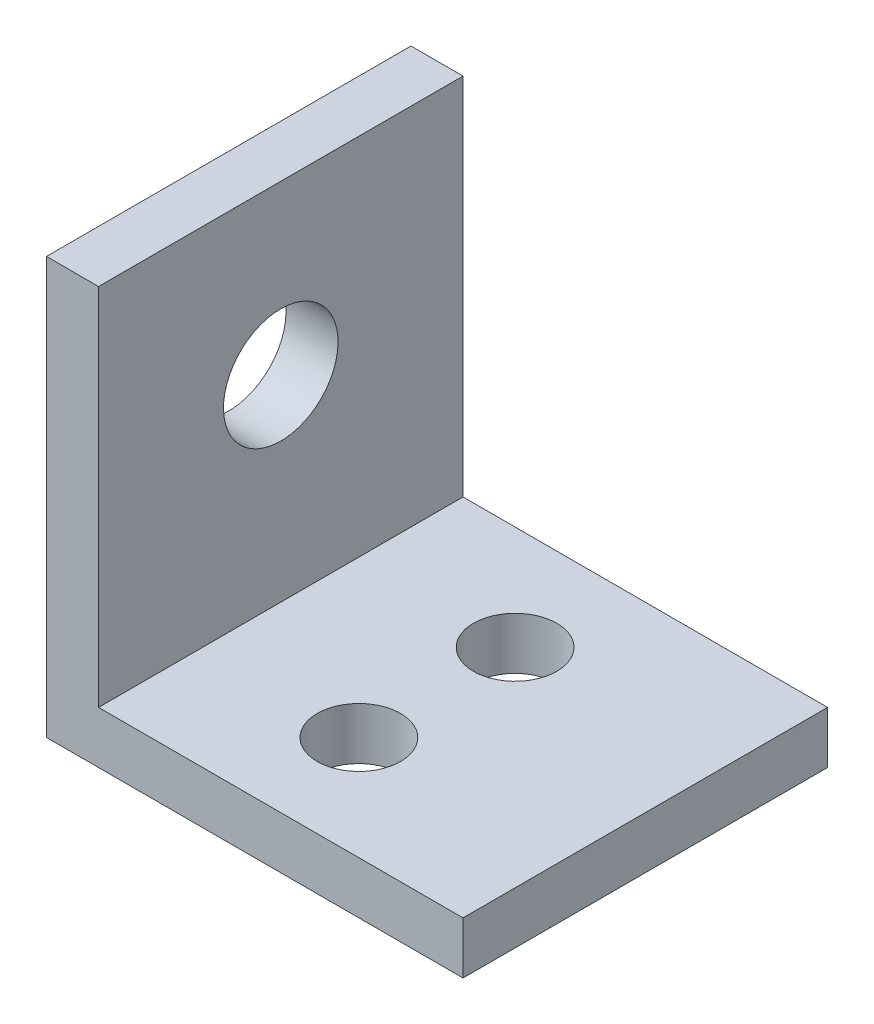
from build123d import *

# Parameters (mm, degrees)
BOSS_EXTRUDE1_DEPTH = 70
SKETCH2_R           = 8
CUT_EXTRUDE1_DEPTH  = 90
SKETCH3_R           = 11
CUT_EXTRUDE2_DEPTH  = 90


with BuildPart() as part:
    # Sketch1 → Boss-Extrude1 (new body)
    with BuildSketch(Plane.XY):
        Polygon((0, 0), (0, 80), (10, 80), (10, 10), (80, 10), (80, 0), align=None)
    extrude(amount=BOSS_EXTRUDE1_DEPTH)

    # Sketch2 → Cut-Extrude1 (cut)
    with BuildSketch(Plane(origin=(0, 10, 0), x_dir=(1, 0, 0), z_dir=(0, 1, 0))):
        with Locations(Location((40, -20, 0), (0, 0, 270))):
            Circle(SKETCH2_R)
        with Locations(Location((40, -50, 0), (0, 0, 270))):
            Circle(SKETCH2_R)
    extrude(amount=-CUT_EXTRUDE1_DEPTH, mode=Mode.SUBTRACT)

    # Sketch3 → Cut-Extrude2 (cut)
    with BuildSketch(Plane(origin=(10, 0, 0), x_dir=(0, 0, -1), z_dir=(1, 0, 0))):
        with Locations(Location((-35, 47.792350155, 0), (0, 0, 90))):
            Circle(SKETCH3_R)
    extrude(amount=-CUT_EXTRUDE2_DEPTH, mode=Mode.SUBTRACT)


solid = part.part
